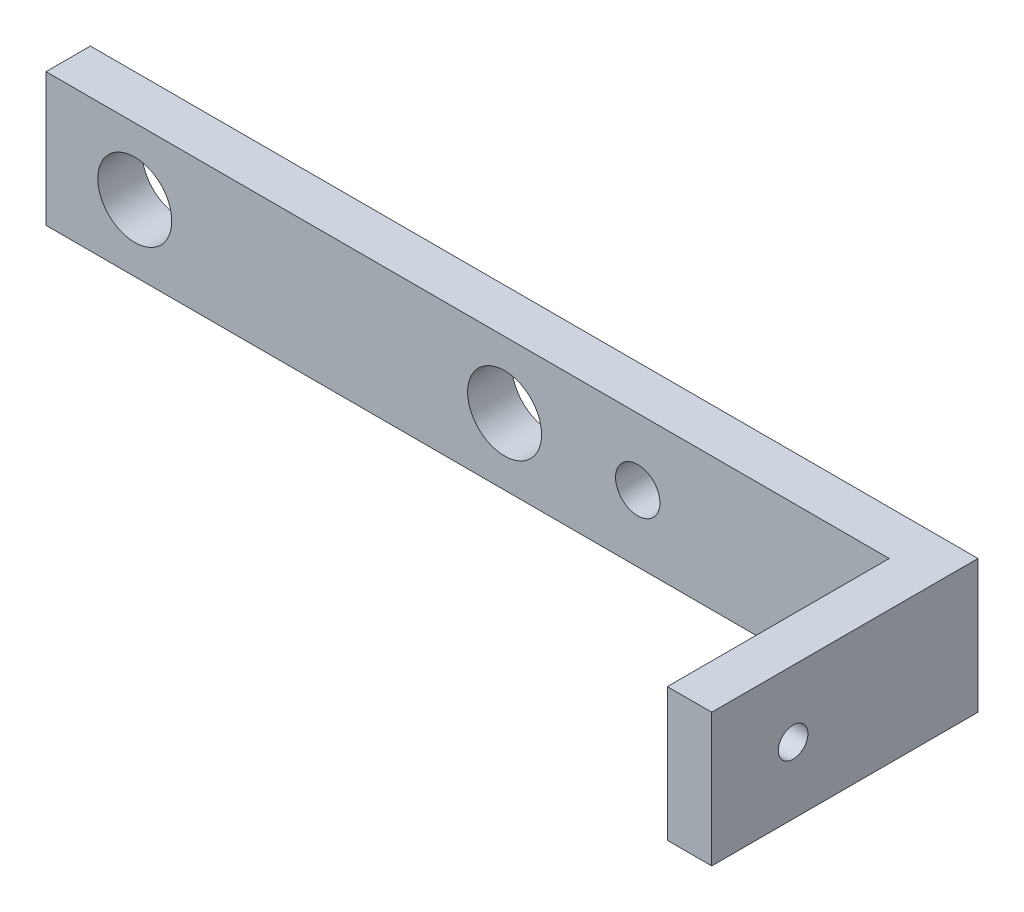
from build123d import *

# Parameters (mm, degrees)
SKETCH_1_W          = 95
SKETCH_1_H          = 18
EXTRUDE_1_DEPTH     = 6
SKETCH_2_R          = 5
CUT_EXTRUDE_1_DEPTH = 6
SKETCH_5_R          = 3
CUT_EXTRUDE_3_DEPTH = 10
SKETCH_6_W          = 6
SKETCH_6_H          = 18
EXTRUDE_3_DEPTH     = 25
SKETCH_7_W          = 6
SKETCH_7_H          = 18
EXTRUDE_4_DEPTH     = 30
SKETCH_8_R          = 2
CUT_EXTRUDE_4_DEPTH = 20


with BuildPart() as part:
    # 草图1 → 凸台-拉伸1 (new body)
    with BuildSketch(Plane.XY):
        Rectangle(SKETCH_1_W, SKETCH_1_H)
    extrude(amount=EXTRUDE_1_DEPTH)

    # 草图2 → 切除-拉伸1 (cut)
    with BuildSketch(Plane.XY.offset(6)):
        with Locations((-35.5, 0)):
            Circle(SKETCH_2_R)
        with Locations((14.5, 0)):
            Circle(SKETCH_2_R)
    extrude(amount=-CUT_EXTRUDE_1_DEPTH, mode=Mode.SUBTRACT)

    # 草图5 → 切除-拉伸3 (cut)
    with BuildSketch(Plane(origin=(0, 0, 0), x_dir=(-1, 0, 0), z_dir=(0, 0, -1))):
        with Locations((-32.5, 0)):
            Circle(SKETCH_5_R)
    extrude(amount=-CUT_EXTRUDE_3_DEPTH, mode=Mode.SUBTRACT)

    # 草图6 → 凸台-拉伸3 (add)
    with BuildSketch(Plane(origin=(47.5, 0, 0), x_dir=(0, 0, -1), z_dir=(1, 0, 0))):
        with Locations((-3, 0)):
            Rectangle(SKETCH_6_W, SKETCH_6_H)
    extrude(amount=EXTRUDE_3_DEPTH)

    # 草图7 → 凸台-拉伸4 (add)
    with BuildSketch(Plane.XY.offset(6)):
        with Locations((69.5, 0)):
            Rectangle(SKETCH_7_W, SKETCH_7_H)
    extrude(amount=EXTRUDE_4_DEPTH)

    # 草图8 → 切除-拉伸4 (cut)
    with BuildSketch(Plane(origin=(72.5, 0, 0), x_dir=(0, 0, -1), z_dir=(1, 0, 0))):
        with Locations((-25, 0)):
            Circle(SKETCH_8_R)
    extrude(amount=-CUT_EXTRUDE_4_DEPTH, mode=Mode.SUBTRACT)


solid = part.part
